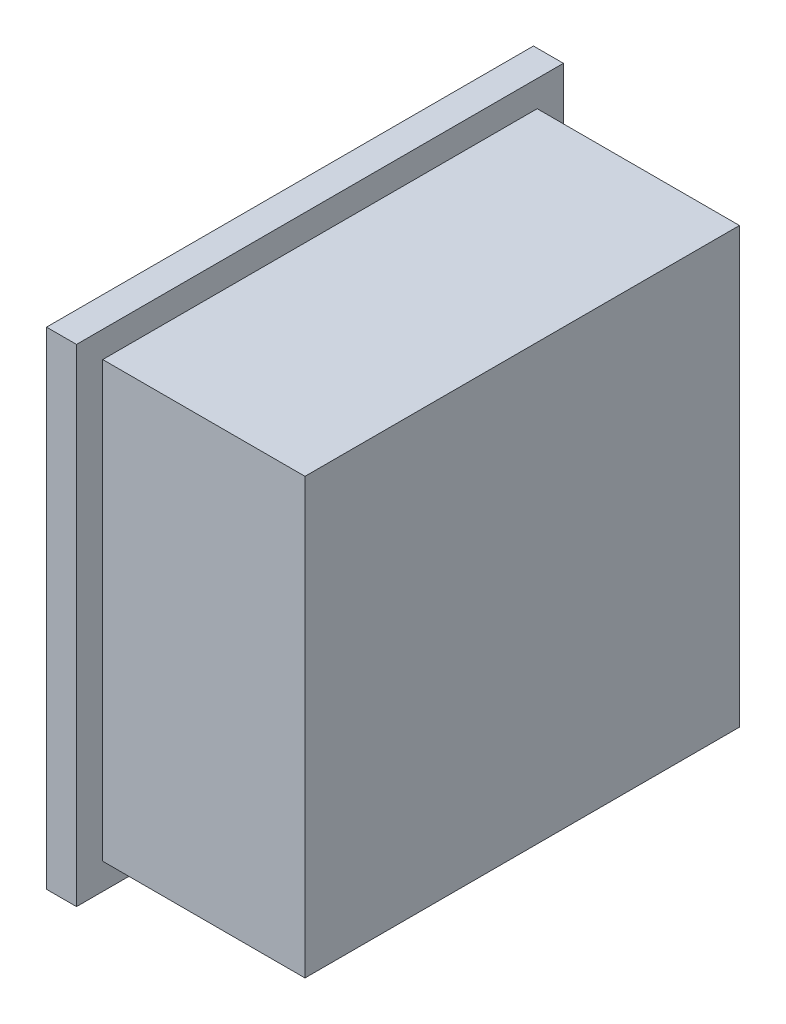
SolidWorks part; units mm, degrees
ref_plane "前视基准面" through (0, 0, 0) normal (0, 0, 1) x (1, 0, 0)
ref_plane "上视基准面" through (0, 0, 0) normal (0, 1, 0) x (1, 0, 0)
ref_plane "右视基准面" through (0, 0, 0) normal (1, 0, 0) x (0, 0, -1)
sketch "草图1" plane through (0, 0, 0) normal (1, 0, 0) x (0, 0, -1)
  line L1 (-65, 65) -> (65, 65)
  line L2 (-65, 65) -> (-65, -65)
  line L3 (-65, -65) -> (65, -65)
  line L4 (65, 65) -> (65, -65)
  line L5 (-65, 65) -> (65, -65) construction
  line L6 (-65, -65) -> (65, 65) construction
  point P0 (0, 0)
  dimension "D1" = 130
  dimension "D2" = 130
extrude "凸台-拉伸1" add sketch "草图1" along normal blind 8
sketch "草图2" plane through (8, 0, 0) normal (1, 0, 0) x (0, 0, -1)
  line L1 (-58, 58) -> (58, 58)
  line L2 (-58, 58) -> (-58, -58)
  line L3 (-58, -58) -> (58, -58)
  line L4 (58, 58) -> (58, -58)
  line L5 (-58, 58) -> (58, -58) construction
  line L6 (-58, -58) -> (58, 58) construction
  point P0 (0, 0)
  dimension "D1" = 116
  dimension "D2" = 116
extrude "凸台-拉伸2" add sketch "草图2" along normal blind 54
sketch "草图3" plane through (0, 0, 0) normal (-1, 0, 0) x (0, 0, 1)
  line L1 (-57.0078, 57.1972) -> (57.0078, 57.1972)
  line L2 (-57.0078, 57.1972) -> (-57.0078, -57.1972)
  line L3 (-57.0078, -57.1972) -> (57.0078, -57.1972)
  line L4 (57.0078, 57.1972) -> (57.0078, -57.1972)
  line L5 (-57.0078, 57.1972) -> (57.0078, -57.1972) construction
  line L6 (-57.0078, -57.1972) -> (57.0078, 57.1972) construction
  point P0 (0, 0)
extrude "切除-拉伸1" cut sketch "草图3" against normal blind 2
